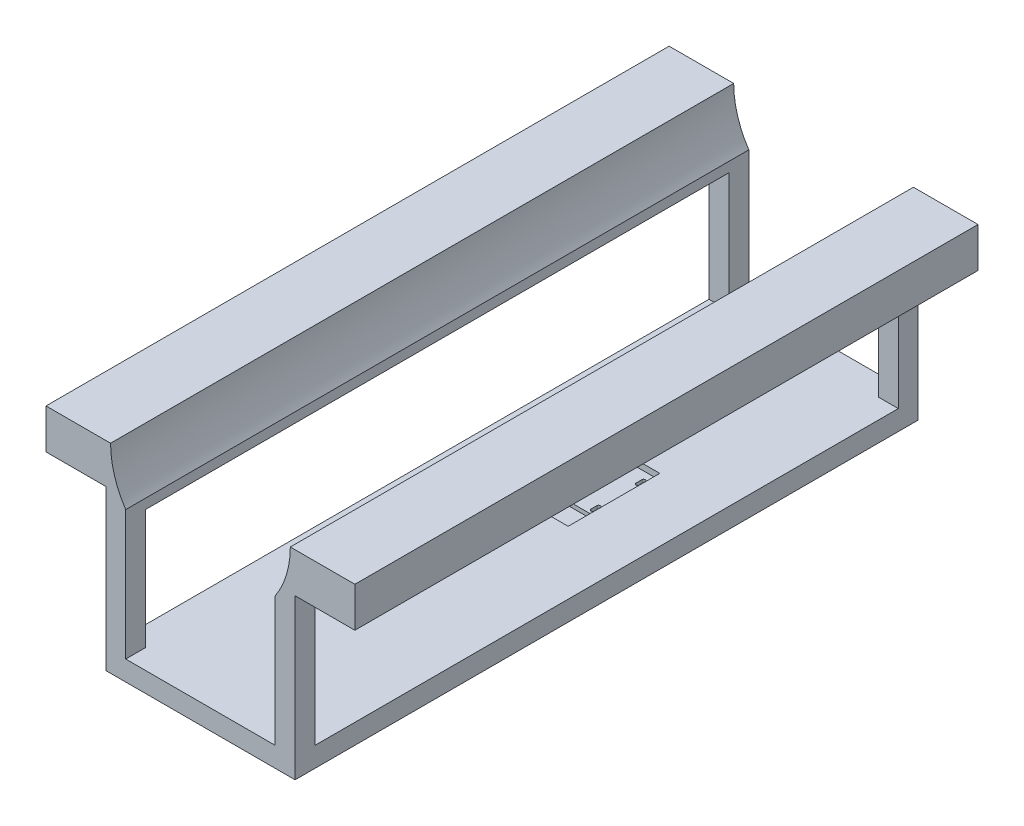
SolidWorks part; units mm, degrees
ref_plane "前视基准面" through (0, 0, 0) normal (0, 0, 1) x (1, 0, 0)
ref_plane "上视基准面" through (0, 0, 0) normal (0, 1, 0) x (1, 0, 0)
ref_plane "右视基准面" through (0, 0, 0) normal (1, 0, 0) x (0, 0, -1)
other "Configuration Table"
sketch "草图1" plane through (0, 0, 0) normal (0, 0, 1) x (1, 0, 0)
  circle A0 centre (0, 0) radius 450 construction
  circle A1 centre (0, 0) radius 37.5
  dimension "D1" = 900
  dimension "D2" = 75
sketch "草图2" plane through (0, 0, 0) normal (0, 1, 0) x (1, 0, 0)
  line L1 (-475, -1563.5) -> (475, -1563.5)
  line L2 (-475, -1563.5) -> (-475, 1563.5)
  line L3 (-475, 1563.5) -> (475, 1563.5)
  line L4 (475, -1563.5) -> (475, 1563.5)
  line L5 (-475, -1563.5) -> (475, 1563.5) construction
  line L6 (-475, 1563.5) -> (475, -1563.5) construction
  point P0 (0, 0)
  dimension "D1" = 950
  dimension "D2" = 3127
extrude "凸台-拉伸1" add sketch "草图2" against normal blind 1000 contours L4 L3 L2 L1
sketch "草图4" plane through (0, 0, 1563.5) normal (0, 0, 1) x (1, 0, 0)
  line L0 (-475, 0) -> (475, 0) construction
  circle A0 centre (0, 0) radius 451
  dimension "D1" = 902
extrude "切除-拉伸1" cut sketch "草图4" against normal blind 3708 contours A0
sketch "草图6" plane through (0, 0, 1563.5) normal (0, 0, 1) x (1, 0, 0)
  line L0 (-475, 0) -> (-775, 0)
  line L1 (-775, 0) -> (-775, -200)
  line L2 (-775, -200) -> (-475, -200)
  line L3 (-475, -1000) -> (-475, 0) construction
  line L4 (-475, -200) -> (-475, 0)
  line L5 (0, 0) -> (0, -450) construction
  line L6 (475, -200) -> (475, 0)
  line L7 (775, -200) -> (475, -200)
  line L8 (775, 0) -> (775, -200)
  line L9 (475, 0) -> (775, 0)
  circle A0 centre (0, 0) radius 450 construction
  point P4 (-475, -100)
  dimension "D1" = 200
  dimension "D2" = 300
extrude "凸台-拉伸2" add sketch "草图6" against normal up to surface (3127 mm away) up to face at (0, -408.5, -1563.5)
sketch "草图9" plane through (0, 0, 1563.5) normal (0, 0, 1) x (1, 0, 0)
  line L0 (475, -1000) -> (475, -200) construction
  line L1 (-375, -550) -> (375, -550)
  line L2 (-375, -550) -> (-375, -900)
  line L3 (-375, -900) -> (375, -900)
  line L4 (375, -550) -> (375, -900)
  line L5 (-475, -1000) -> (475, -1000) construction
  line L6 (-475, -1000) -> (-475, -200) construction
  dimension "D1" = 100
  dimension "D2" = 100
  dimension "D3" = 350
  dimension "D4" = 100
extrude "切除-拉伸2" cut sketch "草图9" against normal blind 3708 contours L4 L3 L2 L1
sketch "草图10" plane through (0, -900, 0) normal (0, 1, 0) x (1, 0, 0)
  line L4 (-375, 1563.5) -> (-375, -1563.5)
  line L5 (-375, -1563.5) -> (375, -1563.5)
  line L6 (375, -1563.5) -> (375, 1563.5)
  line L7 (375, 1563.5) -> (-375, 1563.5)
  line L8 (-375, 1563.5) -> (-375, -1563.5)
  line L9 (-375, -1563.5) -> (375, -1563.5)
  line L10 (375, -1563.5) -> (375, 1563.5)
  line L11 (375, 1563.5) -> (-375, 1563.5)
  dimension "D1" = 0
extrude "切除-拉伸3" cut sketch "草图10" along normal blind 3708 contours L10 L11 L8 L9
sketch "草图11" plane through (0, -900, 0) normal (0, 1, 0) x (1, 0, 0)
  line L0 (-375, 1563.5) -> (375, 1563.5) construction
  line L1 (80, 563.5) -> (158.25, 563.5) construction
  line L2 (80, 563.5) -> (80, 263.5) construction
  line L3 (80, 263.5) -> (158.25, 263.5) construction
  line L4 (158.25, 563.5) -> (158.25, 263.5) construction
  line L5 (110.625, 541.5) -> (110.625, 511.5)
  line L7 (127.625, 511.5) -> (127.625, 541.5)
  line L8 (80, 413.5) -> (158.25, 413.5) construction
  line L9 (127.625, 315.5) -> (127.625, 285.5)
  line L10 (110.625, 285.5) -> (110.625, 315.5)
  line L11 (0, 0) -> (0, 890.2231) construction
  line L12 (-110.625, 285.5) -> (-110.625, 315.5)
  line L13 (-127.625, 315.5) -> (-127.625, 285.5)
  line L14 (-127.625, 511.5) -> (-127.625, 541.5)
  line L15 (-110.625, 541.5) -> (-110.625, 511.5)
  arc A0 (127.625, 541.5) -> (110.625, 541.5) centre (119.125, 541.5) ccw
  arc A1 (110.625, 511.5) -> (127.625, 511.5) centre (119.125, 511.5) ccw
  arc A2 (110.625, 315.5) -> (127.625, 315.5) centre (119.125, 315.5) cw
  arc A3 (127.625, 285.5) -> (110.625, 285.5) centre (119.125, 285.5) cw
  arc A4 (-127.625, 285.5) -> (-110.625, 285.5) centre (-119.125, 285.5) ccw
  arc A5 (-110.625, 315.5) -> (-127.625, 315.5) centre (-119.125, 315.5) ccw
  arc A6 (-110.625, 511.5) -> (-127.625, 511.5) centre (-119.125, 511.5) cw
  arc A7 (-127.625, 541.5) -> (-110.625, 541.5) centre (-119.125, 541.5) cw
  point P5 (119.125, 563.5)
  dimension "D5" = 17
  dimension "D8" = 8.5
  dimension "D1" = 300
  dimension "D2" = 78.25
  dimension "D3" = 1000
  dimension "D4" = 80
  dimension "D6" = 22
  dimension "D7" = 30
extrude "切除-拉伸4" cut sketch "草图11" against normal blind 50
sketch "草图12" plane through (0, -900, 0) normal (0, 1, 0) x (1, 0, 0)
  line L0 (80, 263.5) -> (158.25, 263.5) construction
  line L1 (158.25, 563.5) -> (158.25, 263.5) construction
  line L2 (80, 563.5) -> (80, 263.5) construction
  line L3 (80, 563.5) -> (158.25, 563.5) construction
  line L4 (80, 263.5) -> (158.25, 263.5)
  line L5 (158.25, 563.5) -> (158.25, 263.5)
  line L6 (80, 563.5) -> (80, 263.5)
  line L7 (80, 563.5) -> (158.25, 563.5)
  line L8 (0, 0) -> (0, 890.2231) construction
  line L9 (0, 0) -> (0, 890.2231) construction
  line L10 (-80, 563.5) -> (-158.25, 563.5)
  line L11 (-80, 563.5) -> (-80, 263.5)
  line L12 (-158.25, 563.5) -> (-158.25, 263.5)
  line L13 (-80, 263.5) -> (-158.25, 263.5)
extrude "切除-拉伸5" cut sketch "草图12" against normal blind 30
sketch "草图13" plane through (0, -900, 0) normal (0, 1, 0) x (1, 0, 0)
  line L0 (158.25, 263.5) -> (158.25, 563.5) construction
  line L1 (80, 563.5) -> (158.25, 563.5)
  line L2 (80, 563.5) -> (80, 583.5)
  line L3 (80, 583.5) -> (158.25, 583.5)
  line L4 (158.25, 563.5) -> (158.25, 583.5)
  line L5 (-80, 263.5) -> (-80, 563.5) construction
  line L6 (-158.25, 563.5) -> (-80, 563.5)
  line L7 (-158.25, 563.5) -> (-158.25, 583.5)
  line L8 (-158.25, 583.5) -> (-80, 583.5)
  line L9 (-80, 563.5) -> (-80, 583.5)
  dimension "D1" = 20
  dimension "D2" = 20
extrude "切除-拉伸6" cut sketch "草图13" against normal blind 30
sketch "草图14" plane through (0, -900, 0) normal (0, 1, 0) x (1, 0, 0)
  line L1 (-80, 583.5) -> (80, 583.5)
  line L2 (-80, 583.5) -> (-80, 263.5)
  line L3 (-80, 263.5) -> (80, 263.5)
  line L4 (80, 583.5) -> (80, 263.5)
extrude "切除-拉伸7" cut sketch "草图14" against normal blind 30 contours L4 L3 L2 L1
sketch "草图15" plane through (475, 0, 0) normal (1, 0, 0) x (0, 0, -1)
  line L0 (1563.5, -1000) -> (1563.5, -200) construction
  line L1 (-1463.5, -300) -> (1463.5, -300)
  line L2 (-1463.5, -300) -> (-1463.5, -900)
  line L3 (-1463.5, -900) -> (1463.5, -900)
  line L4 (1463.5, -300) -> (1463.5, -900)
  line L5 (-1563.5, -1000) -> (-1563.5, -200) construction
  line L6 (-1563.5, -1000) -> (1563.5, -1000) construction
  line L7 (1563.5, -200) -> (-1563.5, -200) construction
  point P6 (1563.5, -600)
  dimension "D1" = 100
  dimension "D2" = 100
  dimension "D3" = 100
  dimension "D4" = 100
extrude "切除-拉伸8" cut sketch "草图15" against normal blind 224 contours L2 L3 L4 L1
mirror "镜向1" about plane through (0, 0, 0) normal (1, 0, 0) of "切除-拉伸8"
sketch "草图16" plane through (0, -900, 0) normal (0, 1, 0) x (1, 0, 0)
  line L0 (158.25, 263.5) -> (158.25, 583.5) construction
  line L1 (-158.25, 263.5) -> (158.25, 263.5)
  line L2 (-158.25, 263.5) -> (-158.25, 123.5)
  line L3 (-158.25, 123.5) -> (158.25, 123.5)
  line L4 (158.25, 263.5) -> (158.25, 123.5)
  dimension "D1" = 140
extrude "切除-拉伸9" cut sketch "草图16" against normal blind 50 contours L4 L3 L2 L1
